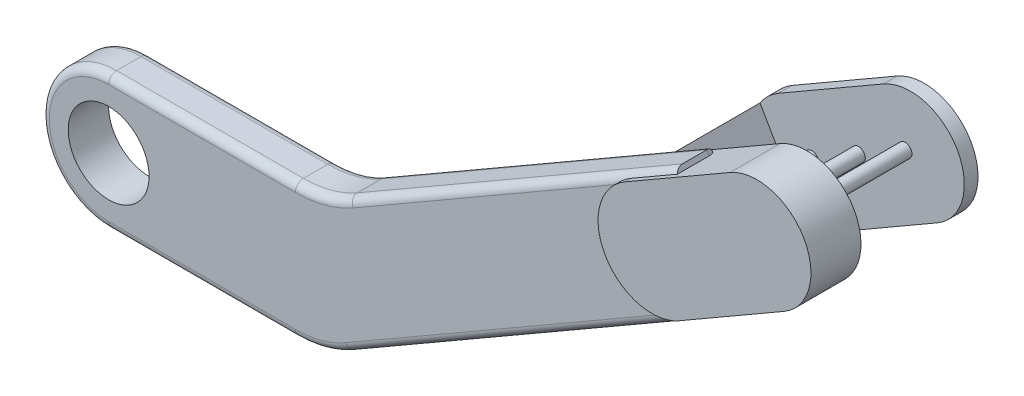
from build123d import *

# Parameters (mm, degrees)
BOSS_EXTRUDE1_DEPTH      = 15
FILLET1_R                = 3
SKETCH2_R                = 15
CUT_EXTRUDE1_DEPTH       = 253.670657786
BOSS_EXTRUDE2_DEPTH      = 45
BOSS_EXTRUDE2_DEPTH_BACK = 17
SKETCH6_W                = 83.616638364
SKETCH6_H                = 38.333633137
CUT_EXTRUDE3_DEPTH       = 289.058075248
SKETCH8_R                = 2.5
BOSS_EXTRUDE3_DEPTH      = 38
LPATTERN1_COUNT          = 3
LPATTERN1_PITCH          = 20


with BuildPart() as part:
    # Sketch1 → Boss-Extrude1 (new body)
    with BuildSketch(Plane.XY):
        with BuildLine():
            Line((0, 25), (69.282032303, 25))
            ThreePointArc((69.282032303, 25), (79.634794107, 26.362966948), (89.282032303, 30.358983849))
            Line((89.282032303, 30.358983849), (209.903810568, 100))
            Line((209.903810568, 100), (231.554445662, 62.5))
            Line((231.554445662, 62.5), (89.282032303, -19.641016151))
            ThreePointArc((89.282032303, -19.641016151), (79.634794107, -23.637033052), (69.282032303, -25))
            Line((69.282032303, -25), (0, -25))
            ThreePointArc((0, -25), (-25, 0), (0, 25))
        make_face()
    extrude(amount=BOSS_EXTRUDE1_DEPTH)

    # Fillet1
    fillet1_edges = [part.edges().sort_by_distance(p)[0] for p in [
        (160.418238983, 21.429491924, 0),
        (79.634794107, -23.637033052, 0),
        (34.641016151, -25, 0),
        (-25, 0, 0),
        (79.634794107, -23.637033052, 15),
        (160.418238983, 21.429491924, 15),
        (149.592921435, 65.179491924, 15),
        (79.634794107, 26.362966948, 15),
        (34.641016151, 25, 15),
        (-25, 0, 15),
        (34.641016151, 25, 0),
        (34.641016151, -25, 15),
        (79.634794107, 26.362966948, 0),
        (149.592921435, 65.179491924, 0),
        (220.729128115, 81.25, 0),
    ]]
    fillet(fillet1_edges, radius=FILLET1_R)

    # Sketch2 → Cut-Extrude1 (cut, through all)
    with BuildSketch(Plane.XY.offset(15)):
        Circle(SKETCH2_R)
    extrude(amount=-CUT_EXTRUDE1_DEPTH, mode=Mode.SUBTRACT)

    # Sketch3 → Boss-Extrude2 (add, two sides: drawn at the far end of the back side and taken through both)
    with BuildSketch(Plane(origin=(0, 0, 0), x_dir=(-1, 0, 0), z_dir=(0, 0, -1)).offset(-BOSS_EXTRUDE2_DEPTH_BACK)):
        with BuildLine():
            Line((-232.55316524, 111.042650187), (-193.582022069, 88.542650187))
            ThreePointArc((-193.582022069, 88.542650187), (-186.261513994, 61.222142112), (-213.582022069, 53.901634036))
            Line((-213.582022069, 53.901634036), (-252.55316524, 76.401634036))
            ThreePointArc((-252.55316524, 76.401634036), (-259.873673315, 103.722142112), (-232.55316524, 111.042650187))
        make_face()
    extrude(amount=BOSS_EXTRUDE2_DEPTH + BOSS_EXTRUDE2_DEPTH_BACK)

    # Sketch6 → Cut-Extrude3 (cut, through all)
    with BuildSketch(Plane(origin=(10.055413327, -17.416486774, 0), x_dir=(0.8660254037844389, 0.4999999999999995, 0), z_dir=(-0.4999999999999995, 0.8660254037844389, 0))):
        with Locations((244.569446826, 20.732918796)):
            Rectangle(SKETCH6_W, SKETCH6_H)
    extrude(amount=-CUT_EXTRUDE3_DEPTH, mode=Mode.SUBTRACT)

    # Sketch8 → Boss-Extrude3 (add)
    with BuildSketch(Plane.XY.offset(-39.899735364)):
        with Locations(Location((240.638883171, 93.826084401, 0), (0, 0, 180))):
            Circle(SKETCH8_R)
    boss_extrude3 = extrude(amount=BOSS_EXTRUDE3_DEPTH)

    # LPattern1: Boss-Extrude3 ×3
    with Locations(*[Vector(-0.8660254037844388, -0.49999999999999983, 0) * (i * LPATTERN1_PITCH) for i in range(1, LPATTERN1_COUNT)]):
        add(boss_extrude3)


solid = part.part
